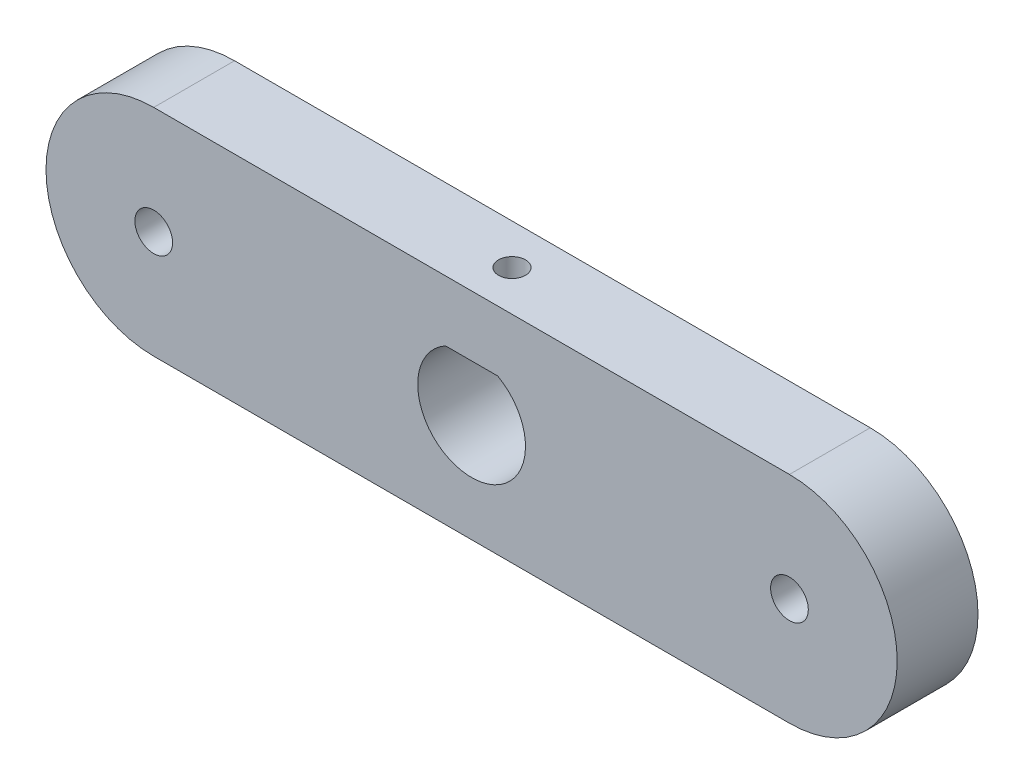
SolidWorks part; units mm, degrees
material "1060 合金"
ref_plane "前视基准面" through (0, 0, 0) normal (0, 0, 1) x (1, 0, 0)
ref_plane "上视基准面" through (0, 0, 0) normal (0, 1, 0) x (1, 0, 0)
ref_plane "右视基准面" through (0, 0, 0) normal (1, 0, 0) x (0, 0, -1)
sketch "草图1" plane through (0, 0, 0) normal (0, 0, 1) x (1, 0, 0)
  line L0 (-23.6, 0) -> (23.6, 0) construction
  line L1 (-23.6, 8) -> (23.6, 8)
  line L2 (-23.6, -8) -> (23.6, -8)
  arc A0 (-23.6, 8) -> (-23.6, -8) centre (-23.6, 0) ccw
  arc A1 (23.6, -8) -> (23.6, 8) centre (23.6, 0) ccw
  circle A2 centre (0, 0) radius 4
  point P2 (0, 0)
  dimension "D1" = 8
  dimension "D2" = 47.2
extrude "凸台-拉伸1" add sketch "草图1" along normal blind 6
sketch "草图2" plane through (0, 0, 6) normal (0, 0, 1) x (1, 0, 0)
  circle A0 centre (-23.6, 0) radius 1.4
  circle A1 centre (23.6, 0) radius 1.4
extrude "切除-拉伸1" cut sketch "草图2" against normal through all
sketch "草图3" plane through (0, 8, 0) normal (0, 1, 0) x (1, 0, 0)
  line L0 (-23.6, -3) -> (23.6, -3) construction
  line L1 (-23.6, -6) -> (-23.6, 0) construction
  line L2 (23.6, -6) -> (23.6, 0) construction
  circle A0 centre (0, -3) radius 1
extrude "切除-拉伸2" cut sketch "草图3" against normal blind 5
sketch "草图4" plane through (0, 0, 0) normal (0, 0, -1) x (-1, 0, 0)
  line L0 (0, 4) -> (0, 2) construction
  line L2 (-2.4801, 4.5) -> (2.4801, 4.5)
  line L3 (-2.4801, 4.5) -> (-2.4801, 3.5)
  line L4 (-2.4801, 3.5) -> (2.4801, 3.5)
  line L5 (2.4801, 4.5) -> (2.4801, 3.5)
  line L6 (-2.4801, 4.5) -> (2.4801, 3.5) construction
  line L7 (-2.4801, 3.5) -> (2.4801, 4.5) construction
  circle A0 centre (0, 0) radius 4 construction
extrude "凸台-拉伸2" add sketch "草图4" against normal up to surface (6 mm away) up to face at (-22.2, 0, 6)
